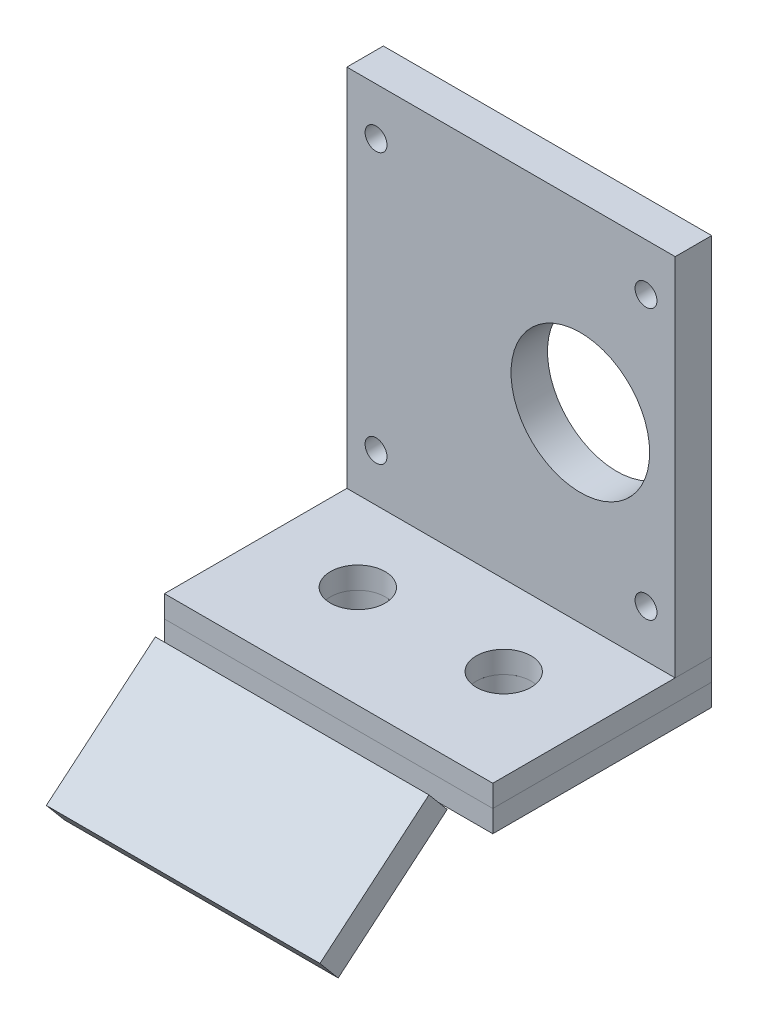
from build123d import *

# Parameters (mm, degrees)
SKETCH_1_W          = 90
SKETCH_1_H          = 100
SKETCH_1_R          = 19
SKETCH_1_R_2        = 3
EXTRUDE_1_DEPTH     = 10
SKETCH_2_W          = 90
SKETCH_2_H          = 60
EXTRUDE_2_DEPTH     = 6
SKETCH_3_W          = 90
SKETCH_3_H          = 60
EXTRUDE_3_DEPTH     = 6
SKETCH_4_R          = 7.5
CUT_EXTRUDE_1_DEPTH = 135.792433022
EXTRUDE_1_2_DEPTH   = 75
SKETCH_6_W          = 75
SKETCH_6_H          = 7.778619134
EXTRUDE_4_DEPTH     = 35


with BuildPart() as part:
    # 草图1 → Extrude 1 (new body)
    with BuildSketch(Plane.XY):
        Rectangle(SKETCH_1_W, SKETCH_1_H)
        with Locations((19, 0)):
            Circle(SKETCH_1_R, mode=Mode.SUBTRACT)
        with Locations((-37, 37)):
            Circle(SKETCH_1_R_2, mode=Mode.SUBTRACT)
        with Locations(Location((37, 37, 0), (0, 0, 180))):
            Circle(SKETCH_1_R_2, mode=Mode.SUBTRACT)
        with Locations((37, -37)):
            Circle(SKETCH_1_R_2, mode=Mode.SUBTRACT)
        with Locations(Location((-37, -37, 0), (0, 0, 180))):
            Circle(SKETCH_1_R_2, mode=Mode.SUBTRACT)
    extrude(amount=EXTRUDE_1_DEPTH)


with BuildPart() as body_2:
    # 草图2 → 凸台-拉伸2 (new body)
    with BuildSketch(Plane(origin=(0, -50, 0), x_dir=(1, 0, 0), z_dir=(0, 1, 0))):
        with Locations((0, -30)):
            Rectangle(SKETCH_2_W, SKETCH_2_H)
    extrude(amount=-EXTRUDE_2_DEPTH)


with BuildPart() as body_3:
    # 草图3 → 凸台-拉伸3 (new body)
    with BuildSketch(Plane(origin=(0, -56, 0), x_dir=(-1, 0, 0), z_dir=(0, -1, 0))):
        with Locations((0, -30)):
            Rectangle(SKETCH_3_W, SKETCH_3_H)
    extrude(amount=EXTRUDE_3_DEPTH)


with BuildPart() as cut_extrude_1_tool:
    # 草图4 → 切除-拉伸1 (new, through all)
    with BuildSketch(Plane(origin=(0, -62, 0), x_dir=(-1, 0, 0), z_dir=(0, -1, 0))):
        with Locations(Location((-20, -32, 0), (0, 0, 180))):
            Circle(SKETCH_4_R)
        with Locations(Location((20, -32, 0), (0, 0, 180))):
            Circle(SKETCH_4_R)
    extrude(amount=-CUT_EXTRUDE_1_DEPTH)


with BuildPart() as body_2_1:
    add(body_2.part)

    # 切除-拉伸1: cut by cut_extrude_1_tool
    add(cut_extrude_1_tool.part, mode=Mode.SUBTRACT)


with BuildPart() as body_3_1:
    add(body_3.part)

    # 切除-拉伸1: cut by cut_extrude_1_tool
    add(cut_extrude_1_tool.part, mode=Mode.SUBTRACT)


with BuildPart() as body_4:
    # 草图5 → Extrude 1 2 (new body)
    with BuildSketch(Plane(origin=(-45, 0, 0), x_dir=(0, 0, -1), z_dir=(1, 0, 0))):
        Polygon((-62.5, -59.020616019), (-57.5, -64.979383981), (-60.564177772, -67.55053442), (-65.564177772, -61.591766457), align=None)
    extrude(amount=EXTRUDE_1_2_DEPTH)

    # 草图6 → 凸台-拉伸4 (add)
    with BuildSketch(Plane(origin=(0, -130.316769058, 7.897053438), x_dir=(-1, 0, 0), z_dir=(0, -0.6427876096865384, 0.7660444431189789))):
        with Locations((7.5, -85.824809787)):
            Rectangle(SKETCH_6_W, SKETCH_6_H)
    extrude(amount=EXTRUDE_4_DEPTH)


solid = Compound([part.part, body_2_1.part, body_3_1.part, body_4.part])
